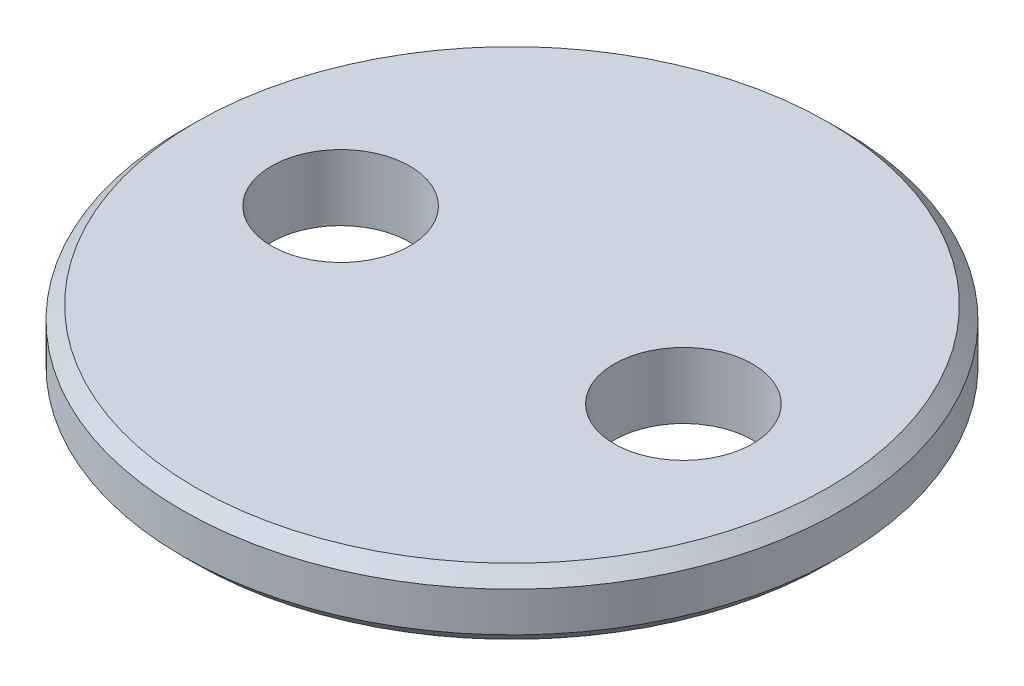
from build123d import *

# Parameters (mm, degrees)
SKETCH1_R           = 25
SKETCH1_R_2         = 5.25
BOSS_EXTRUDE1_DEPTH = 5
CHAMFER1_SIZE       = 1


with BuildPart() as part:
    # Sketch1 → Boss-Extrude1 (new body)
    with BuildSketch(Plane(origin=(0, 0, 0), x_dir=(1, 0, 0), z_dir=(0, 1, 0))):
        with Locations(Location((0, 0, 0), (0, 0, 270))):
            Circle(SKETCH1_R)
        with Locations(Location((-13, 0, 0), (0, 0, 270))):
            Circle(SKETCH1_R_2, mode=Mode.SUBTRACT)
        with Locations(Location((13, 0, 0), (0, 0, 90))):
            Circle(SKETCH1_R_2, mode=Mode.SUBTRACT)
    extrude(amount=BOSS_EXTRUDE1_DEPTH)

    # Chamfer1
    chamfer1_edges = [part.edges().sort_by_distance(p)[0] for p in [
        (0, 0, -25),
        (0, 5, -25),
    ]]
    chamfer(chamfer1_edges, length=CHAMFER1_SIZE)


solid = part.part
